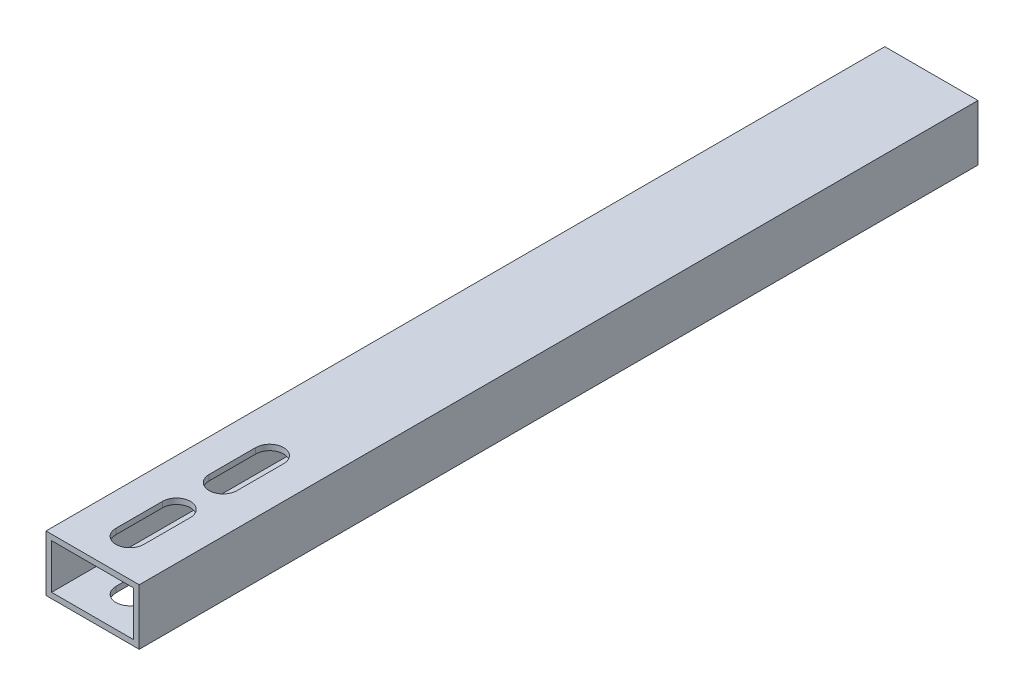
from build123d import *

# Parameters (mm, degrees)
SKETCH_1_W          = 50
SKETCH_1_H          = 30
SKETCH_1_W_2        = 44
SKETCH_1_H_2        = 24
EXTRUDE_1_DEPTH     = 450
CUT_EXTRUDE_2_DEPTH = 450
CUT_EXTRUDE_3_DEPTH = 450


with BuildPart() as part:
    # 草图1 → 凸台-拉伸1 (new body)
    with BuildSketch(Plane.XY):
        with Locations((25, 15)):
            Rectangle(SKETCH_1_W, SKETCH_1_H)
        with Locations((25, 15)):
            Rectangle(SKETCH_1_W_2, SKETCH_1_H_2, mode=Mode.SUBTRACT)
    extrude(amount=EXTRUDE_1_DEPTH)

    # 草图2 → 切除-拉伸2 (cut)
    with BuildSketch(Plane.XZ):
        with BuildLine():
            Line((17.5, 430), (17.5, 405))
            ThreePointArc((17.5, 405), (25, 397.5), (32.5, 405))
            Line((32.5, 405), (32.5, 430))
            ThreePointArc((32.5, 430), (25, 437.5), (17.5, 430))
        make_face()
    extrude(amount=-CUT_EXTRUDE_2_DEPTH, mode=Mode.SUBTRACT)

    # 草图4 → 切除-拉伸3 (cut)
    with BuildSketch(Plane.XZ):
        with BuildLine():
            Line((17.5, 380), (17.5, 355))
            ThreePointArc((17.5, 355), (25, 347.5), (32.5, 355))
            Line((32.5, 355), (32.5, 380))
            ThreePointArc((32.5, 380), (25, 387.5), (17.5, 380))
        make_face()
    extrude(amount=-CUT_EXTRUDE_3_DEPTH, mode=Mode.SUBTRACT)


solid = part.part
